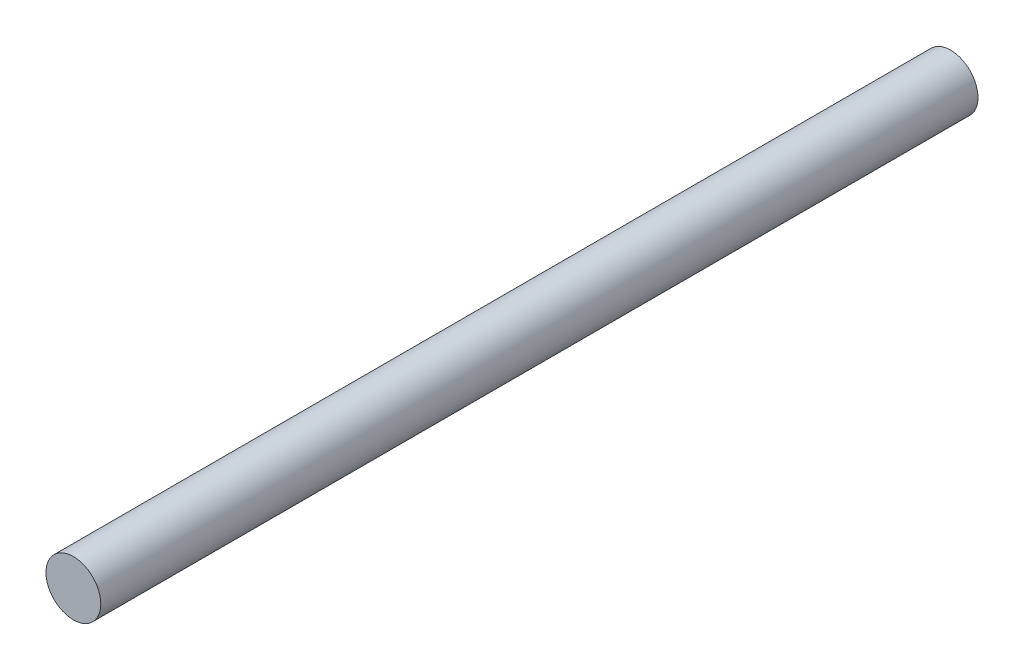
from build123d import *

# Parameters (mm, degrees)
SKETCH_1_R      = 7.5
EXTRUDE_1_DEPTH = 240


with BuildPart() as part:
    # 草图1 → 凸台-拉伸1 (new body)
    with BuildSketch(Plane.XY):
        Circle(SKETCH_1_R)
    extrude(amount=EXTRUDE_1_DEPTH)


solid = part.part
